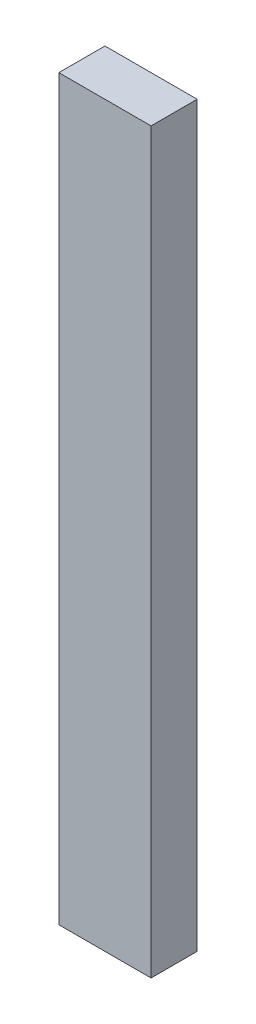
SolidWorks part; units mm, degrees
ref_plane "Plane1" through (0, 0, 0) normal (0, 0, 1) x (1, 0, 0)
ref_plane "Plane2" through (0, 0, 0) normal (0, 1, 0) x (1, 0, 0)
ref_plane "Plane3" through (0, 0, 0) normal (1, 0, 0) x (0, 0, -1)
sketch "Sketch1" plane through (0, 0, 0) normal (0, 0, 1) x (1, 0, 0)
  line L8 (0, -40) -> (0, 40)
  line L9 (0, 40) -> (-10, 40)
  line L10 (-10, 40) -> (-10, -40)
  line L11 (-10, -40) -> (0, -40)
extrude "Base-Extrude" add sketch "Sketch1" along normal blind 5
